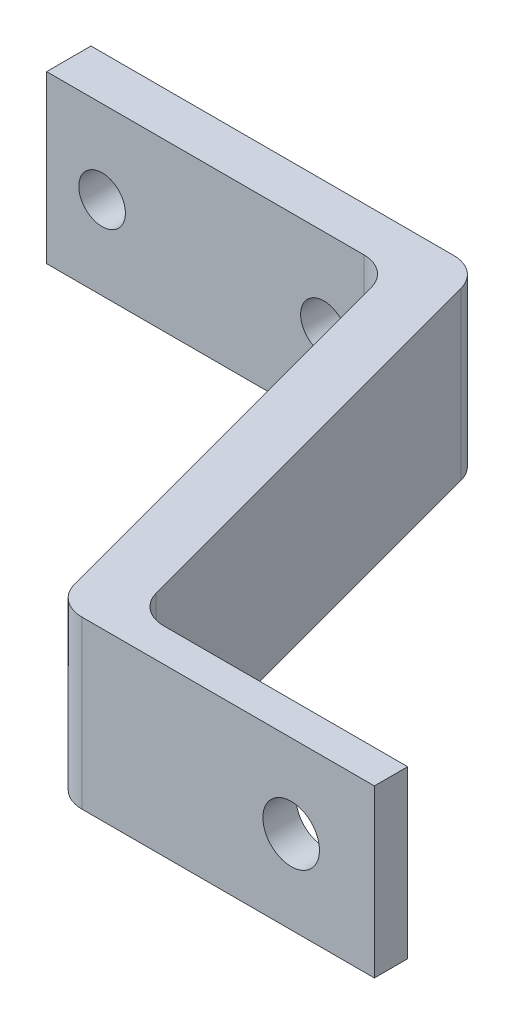
from build123d import *

# Parameters (mm, degrees)
EXTRUDE_1_DEPTH          = 15
CUT_EXTRUDE_1_DEPTH      = 84.464378629
CUT_EXTRUDE_1_DEPTH_BACK = 84.464378629
SKETCH_2_R               = 2.55
SKETCH_2_R_2             = 2.1
FILLET_1_R               = 3


with BuildPart() as part:
    # 草图1 → 凸台-拉伸1 (new body)
    with BuildSketch(Plane(origin=(0, 0, 0), x_dir=(1, 0, 0), z_dir=(0, 1, 0))):
        Polygon((0, 0), (0, -4), (30.895415868, -4), (41.881332757, -45), (70.55, -45), (70.55, -42), (46.253866082, -42), (35, 0), align=None)
    extrude(amount=EXTRUDE_1_DEPTH)

    # 草图2 → 切除-拉伸1 (cut, two sides: drawn at the far end of the back side and taken through both)
    with BuildSketch(Plane(origin=(0, 0, 42), x_dir=(-1, 0, 0), z_dir=(0, 0, -1)).offset(-CUT_EXTRUDE_1_DEPTH_BACK)):
        with Locations((-63.05, 7.5)):
            Circle(SKETCH_2_R)
        with Locations((-25, 7.5)):
            Circle(SKETCH_2_R_2)
        with Locations((-5, 7.5)):
            Circle(SKETCH_2_R_2)
    extrude(amount=CUT_EXTRUDE_1_DEPTH + CUT_EXTRUDE_1_DEPTH_BACK, mode=Mode.SUBTRACT)

    # 圆角1
    fillet_1_edges = [part.edges().sort_by_distance(p)[0] for p in [
        (35, 7.5, 0),
        (46.253866082, 7.5, 42),
        (41.881332757, 7.5, 45),
        (30.895415868, 7.5, 4),
    ]]
    fillet(fillet_1_edges, radius=FILLET_1_R)


solid = part.part
